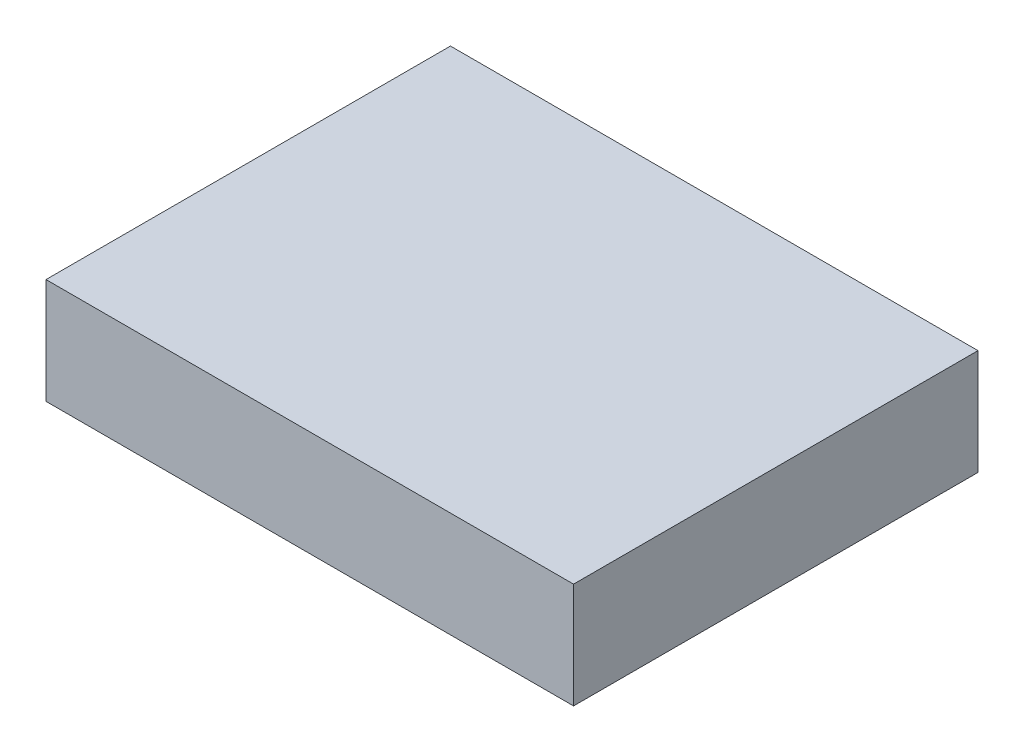
from build123d import *

# Parameters (mm, degrees)
SKETCH1_W           = 60
SKETCH1_H           = 46
BOSS_EXTRUDE1_DEPTH = 12


with BuildPart() as part:
    # Sketch1 → Boss-Extrude1 (new body)
    with BuildSketch(Plane(origin=(0, 0, 0), x_dir=(1, 0, 0), z_dir=(0, 1, 0))):
        with Locations((30, -23)):
            Rectangle(SKETCH1_W, SKETCH1_H)
    extrude(amount=BOSS_EXTRUDE1_DEPTH)


solid = part.part
